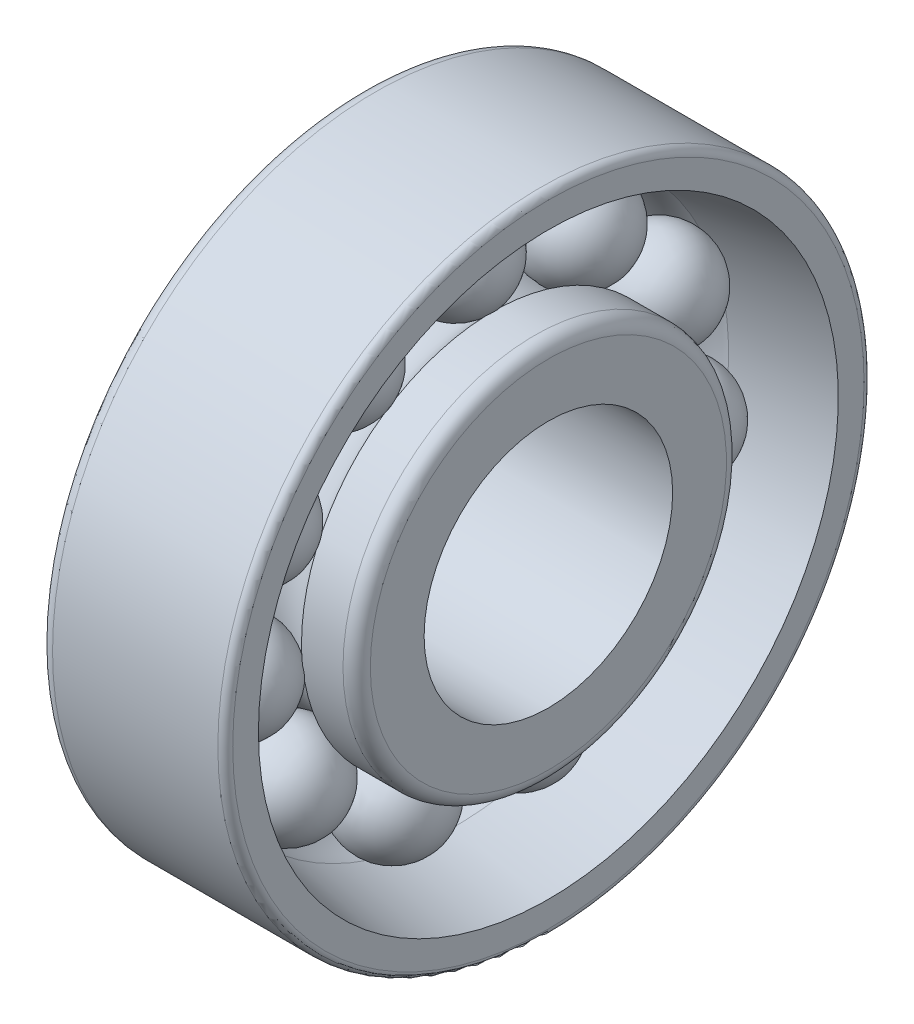
from build123d import *

# Parameters (mm, degrees)
FILLET1_R         = 0.6
FILLET2_R         = 1.1
CIRPATTERN2_COUNT = 11


with BuildPart() as part:
    # Sketch2 → Base-Revolve (revolve)
    with BuildSketch(Plane.XY, mode=Mode.PRIVATE) as base_revolve_sk:
        with BuildLine():
            Line((0, 26), (15, 26))
            Line((15, 26), (15, 23.333333333))
            Line((15, 23.333333333), (7.5, 22))
            ThreePointArc((7.5, 22), (5.809526953, 21.625231148), (4.435822228, 20.571150439))
            Line((4.435822228, 20.571150439), (0, 20.571150439))
            Line((0, 20.571150439), (0, 26))
        make_face()
    revolve(base_revolve_sk.sketch.rotate(Axis((0, 0, 0), (1, 0, 0)), 90), axis=Axis((0, 0, 0), (1, 0, 0)))

    # Sketch3 → Boss-Revolve1 (revolve)
    with BuildSketch(Plane.XY):
        with BuildLine():
            Line((11.55, 18), (3.45, 18))
            ThreePointArc((3.45, 18), (7.5, 22.05), (11.55, 18))
        make_face()
    boss_revolve1 = revolve(axis=Axis((0, 18, 0), (1, 0, 0)))

    # Sketch4 → Boss-Revolve2 (revolve)
    with BuildSketch(Plane.XY, mode=Mode.PRIVATE) as boss_revolve2_sk:
        with BuildLine():
            Line((15, 10), (15, 15.428849561))
            Line((15, 15.428849561), (10.564177772, 15.428849561))
            ThreePointArc((10.564177772, 15.428849561), (7.5, 14), (4.435822228, 15.428849561))
            Line((4.435822228, 15.428849561), (0, 15.428849561))
            Line((0, 15.428849561), (0, 10))
            Line((0, 10), (15, 10))
        make_face()
    revolve(boss_revolve2_sk.sketch.rotate(Axis((0, 0, 0), (1, 0, 0)), 90), axis=Axis((0, 0, 0), (1, 0, 0)))

    # Fillet1
    fillet1_edges = [part.edges().sort_by_distance(p)[0] for p in [
        (15, 0, -26),
    ]]
    fillet(fillet1_edges, radius=FILLET1_R)

    # Fillet2
    fillet2_edges = [part.edges().sort_by_distance(p)[0] for p in [
        (15, 0, -15.428849561),
        (0, 0, -26),
    ]]
    fillet(fillet2_edges, radius=FILLET2_R)

    # CirPattern2: Boss-Revolve1 ×11 about axis
    cirpattern2_axis = Axis((0, 0, 0), (1, 0, 0))
    for i in range(1, CIRPATTERN2_COUNT):
        add(boss_revolve1.rotate(cirpattern2_axis, i * 360 / CIRPATTERN2_COUNT))


solid = part.part
